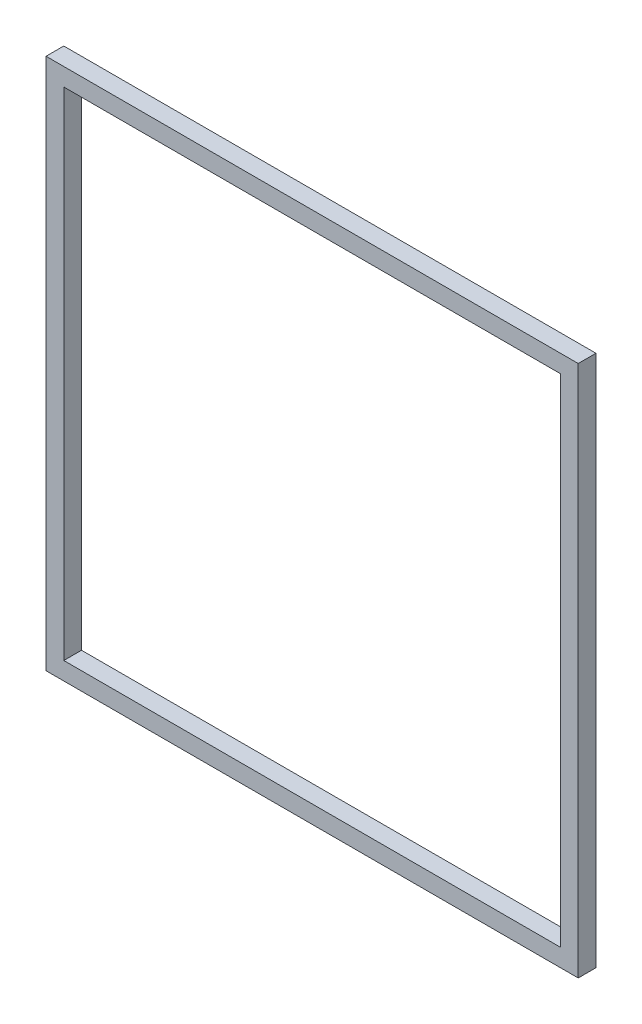
from build123d import *

# Parameters (mm, degrees)
SKETCH_1_W      = 300
SKETCH_1_H      = 300
SKETCH_1_W_2    = 280
SKETCH_1_H_2    = 280
EXTRUDE_1_DEPTH = 5


with BuildPart() as part:
    # 草图1 → 凸台-拉伸1 (new, symmetric)
    with BuildSketch(Plane.XY):
        Rectangle(SKETCH_1_W, SKETCH_1_H)
        Rectangle(SKETCH_1_W_2, SKETCH_1_H_2, mode=Mode.SUBTRACT)
    extrude(amount=EXTRUDE_1_DEPTH, both=True)


solid = part.part
